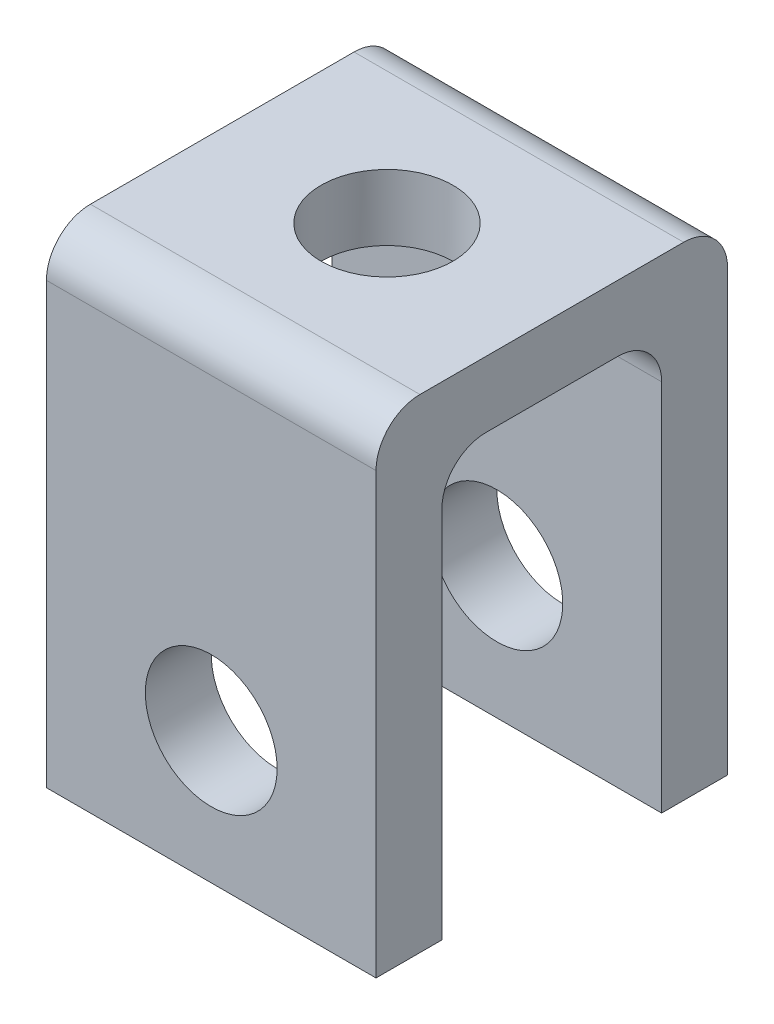
from build123d import *

# Parameters (mm, degrees)
SKETCH1_W           = 15
SKETCH1_H           = 22
SKETCH1_R           = 3
BOSS_EXTRUDE1_DEPTH = 8
SKETCH2_W           = 10
SKETCH2_H           = 19
CUT_EXTRUDE1_DEPTH  = 24.34523506
FILLET1_R           = 2
SKETCH3_R           = 3
CUT_EXTRUDE2_DEPTH  = 18


with BuildPart() as part:
    # Sketch1 → Boss-Extrude1 (new, symmetric)
    with BuildSketch(Plane.XY):
        with Locations((0, 5)):
            Rectangle(SKETCH1_W, SKETCH1_H)
        Circle(SKETCH1_R, mode=Mode.SUBTRACT)
    extrude(amount=BOSS_EXTRUDE1_DEPTH, both=True)

    # Sketch2 → Cut-Extrude1 (cut, through all)
    with BuildSketch(Plane(origin=(7.5, 0, 0), x_dir=(0, 0, -1), z_dir=(1, 0, 0))):
        with Locations((0, 3.5)):
            Rectangle(SKETCH2_W, SKETCH2_H)
    extrude(amount=-CUT_EXTRUDE1_DEPTH, mode=Mode.SUBTRACT)

    # Fillet1
    fillet1_edges = [part.edges().sort_by_distance(p)[0] for p in [
        (0, 16, 8),
        (0, 13, 5),
        (0, 13, -5),
        (0, 16, -8),
    ]]
    fillet(fillet1_edges, radius=FILLET1_R)

    # Sketch3 → Cut-Extrude2 (cut)
    with BuildSketch(Plane(origin=(0, 16, 0), x_dir=(1, 0, 0), z_dir=(0, 1, 0))):
        with Locations(Location((0, 0, 0), (0, 0, 270))):
            Circle(SKETCH3_R)
    extrude(amount=-CUT_EXTRUDE2_DEPTH, mode=Mode.SUBTRACT)


solid = part.part
